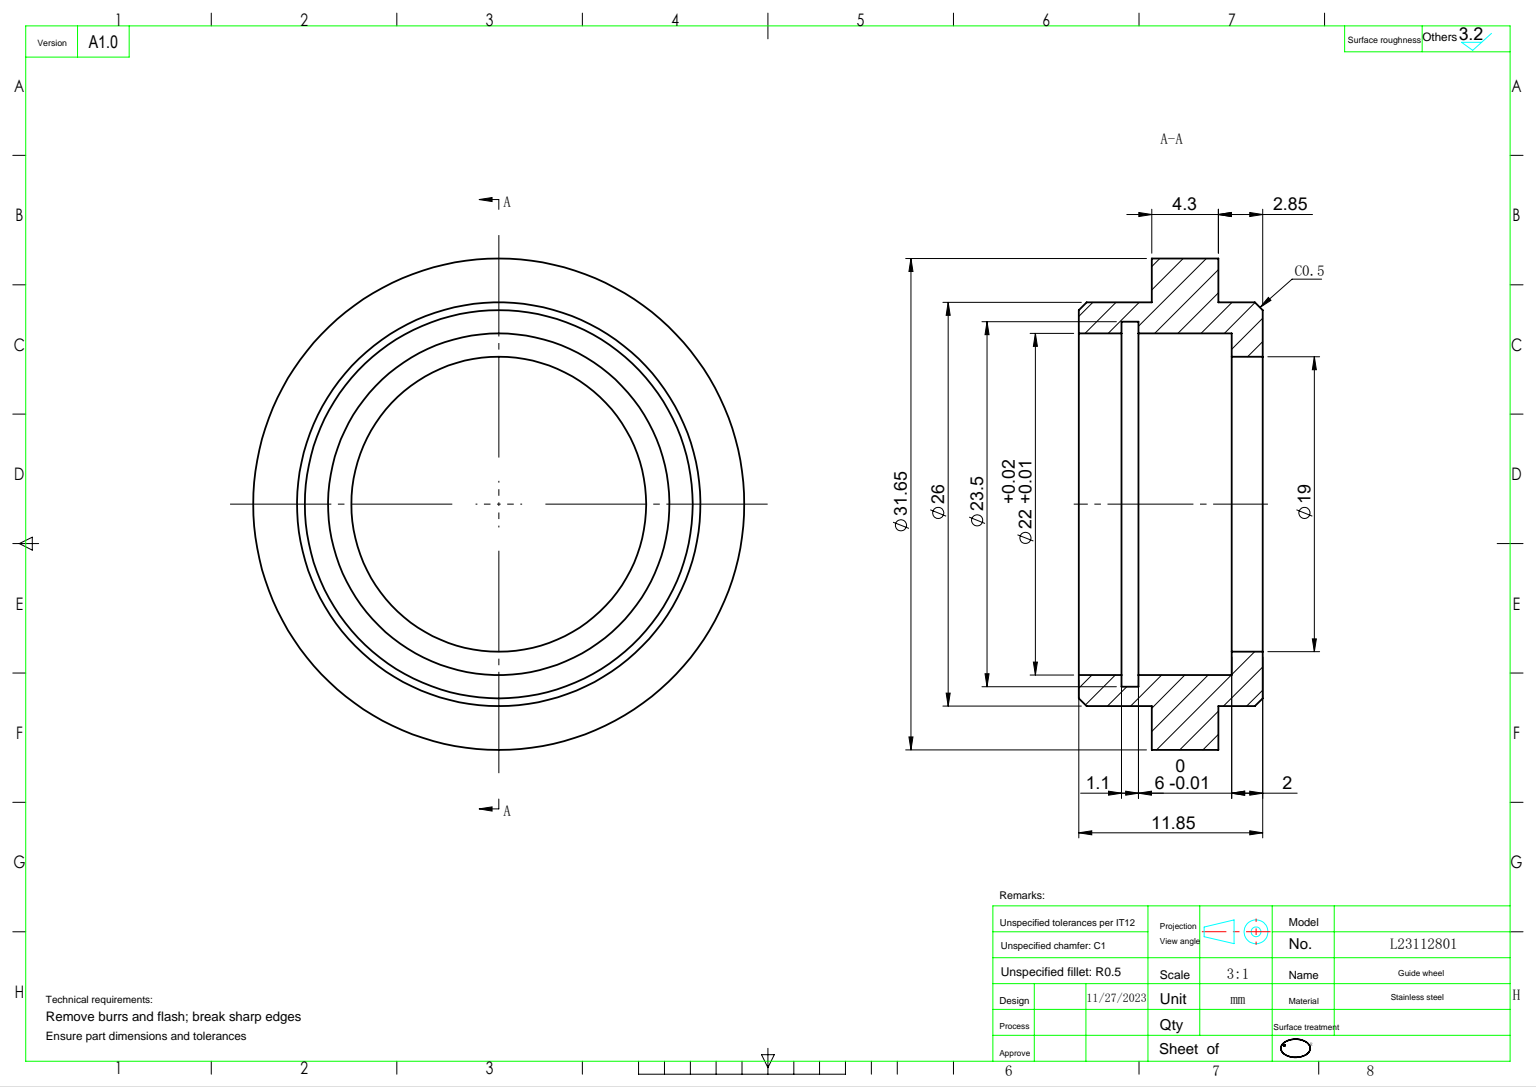
SolidWorks part; units mm, degrees
ref_plane "前视基准面" through (0, 0, 0) normal (0, 0, 1) x (1, 0, 0)
ref_plane "上视基准面" through (0, 0, 0) normal (0, 1, 0) x (1, 0, 0)
ref_plane "右视基准面" through (0, 0, 0) normal (1, 0, 0) x (0, 0, -1)
sketch "草图1" plane through (0, 0, 0) normal (0, 0, 1) x (1, 0, 0)
  line L0 (0, 0) -> (36.0184, 0) construction
  line L1 (0, 9.5) -> (0, 13)
  line L2 (0, 13) -> (2.85, 13)
  line L3 (2.85, 13) -> (2.85, 15.825)
  line L4 (2.85, 15.825) -> (7.15, 15.825)
  line L5 (7.15, 15.825) -> (7.15, 13)
  line L6 (7.15, 13) -> (11.85, 13)
  line L7 (11.85, 13) -> (11.85, 9.5)
  line L8 (11.85, 9.5) -> (0, 9.5)
  dimension "D1" = 19
  dimension "D2" = 26
  dimension "D3" = 31.65
  dimension "D4" = 2.85
  dimension "D5" = 4.3
  dimension "D6" = 11.85
revolve "旋转1" add sketch "草图1" angle 360 about L0
sketch "草图2" plane through (0, 0, 0) normal (1, 0, 0) x (0, 0, -1)
  circle A0 centre (0, 0) radius 11
  dimension "D1" = 22
extrude "切除-拉伸1" cut sketch "草图2" along normal through all from offset 2
sketch "草图3" plane through (2, 0, 0) normal (1, 0, 0) x (0, 0, -1)
  circle A0 centre (0, 0) radius 11.75
  dimension "D1" = 23.5
extrude "切除-拉伸2" cut sketch "草图3" along normal blind 1.1 from offset 6
chamfer "倒角1" distance 0.5 angle 45 2 edges at (11.85, 0, 13) (0, 0, 13)
